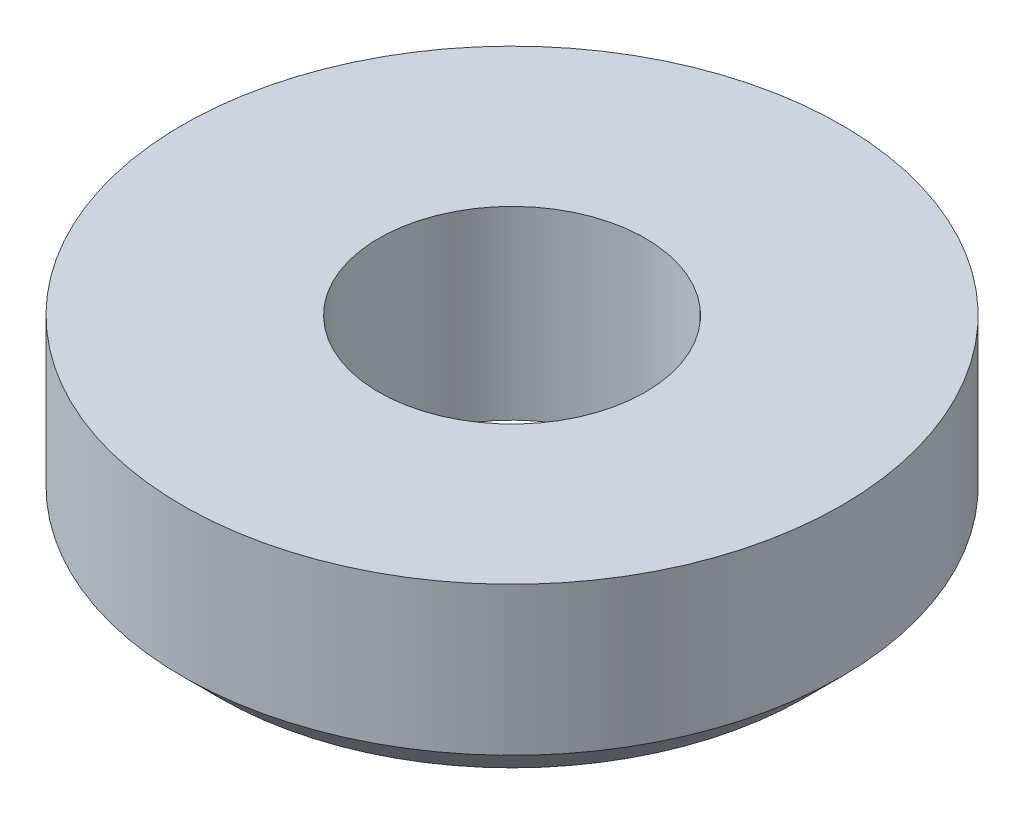
SolidWorks part; units mm, degrees
material "Rubber"
ref_plane "Front Plane" through (0, 0, 0) normal (0, 0, 1) x (1, 0, 0)
ref_plane "Top Plane" through (0, 0, 0) normal (0, 1, 0) x (1, 0, 0)
ref_plane "Right Plane" through (0, 0, 0) normal (1, 0, 0) x (0, 0, -1)
sketch "Sketch1" plane through (0, 0, 0) normal (0, 0, 1) x (1, 0, 0)
  line L0 (0, -964.3541) -> (0, 47253.3518) construction
  line L2 (18, 0) -> (44.5, 0)
  line L3 (18, 0) -> (18, 25)
  line L4 (18, 25) -> (44.5, 25)
  line L5 (44.5, 0) -> (44.5, 25)
  dimension "D1" = 18
  dimension "D2" = 44.5
  dimension "D3" = 25
revolve "Revolve1" add sketch "Sketch1" angle 360 about L0
chamfer "Chamfer1" distance 5 angle 45 1 edges at (44.5, 0, 0)
